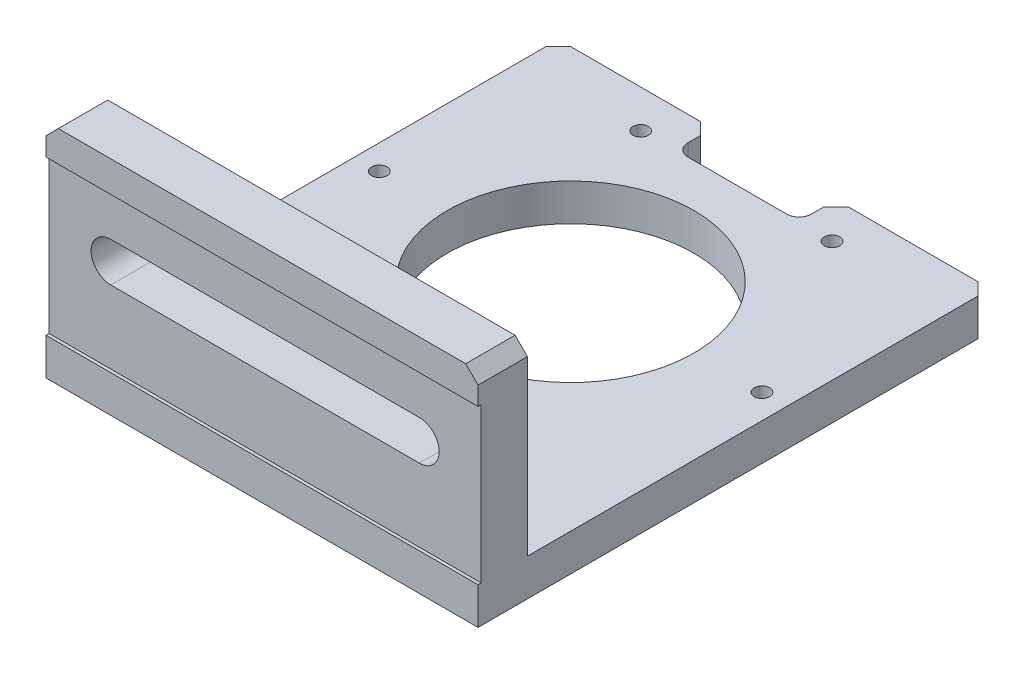
SolidWorks part; units mm, degrees
ref_plane "Front Plane" through (0, 0, 0) normal (0, 0, 1) x (1, 0, 0)
ref_plane "Top Plane" through (0, 0, 0) normal (0, 1, 0) x (1, 0, 0)
ref_plane "Right Plane" through (0, 0, 0) normal (1, 0, 0) x (0, 0, -1)
sketch "Sketch1" plane through (0, 0, 0) normal (0, 1, 0) x (1, 0, 0)
  line L1 (-35, -41.5) -> (35, -41.5)
  line L2 (-35, -41.5) -> (-35, 41.5)
  line L3 (-35, 41.5) -> (35, 41.5)
  line L4 (35, -41.5) -> (35, 41.5)
  line L5 (-35, -41.5) -> (35, 41.5) construction
  line L6 (-35, 41.5) -> (35, -41.5) construction
  point P0 (0, 0)
  dimension "D1" = 70
  dimension "D2" = 83
extrude "Boss-Extrude1" add sketch "Sketch1" along normal blind 6
sketch "Sketch2" plane through (0, 6, 0) normal (0, 1, 0) x (1, 0, 0)
  line L0 (35, -41.5) -> (35, 41.5) construction
  line L1 (-35, -41.5) -> (35, -41.5)
  line L2 (-35, -41.5) -> (-35, -33.5)
  line L3 (-35, -33.5) -> (35, -33.5)
  line L4 (35, -41.5) -> (35, -33.5)
  dimension "D1" = 8
extrude "Boss-Extrude2" add sketch "Sketch2" along normal blind 30
sketch "Sketch3" plane through (0, 0, 0) normal (0, -1, 0) x (1, 0, 0)
  line L0 (-35, 41.5) -> (35, 41.5) construction
  line L1 (-35, -41.5) -> (-35, 41.5) construction
  circle A0 centre (0, -8.5) radius 20
  dimension "D1" = 50
  dimension "D3" = 40
  dimension "D2" = 35
extrude "Cut-Extrude1" cut sketch "Sketch3" against normal blind 20
sketch "Sketch4" plane through (0, 6, 0) normal (0, 1, 0) x (1, 0, 0)
  line L0 (35, 41.5) -> (-35, 41.5) construction
  line L1 (-10, 47.5192) -> (10, 47.5192)
  line L2 (-10, 47.5192) -> (-10, 35.5)
  line L3 (-10, 35.5) -> (10, 35.5)
  line L4 (10, 47.5192) -> (10, 35.5)
  line L5 (-35, 41.5) -> (-35, -33.5) construction
  line L6 (35, -33.5) -> (35, 41.5) construction
  dimension "D1" = 6
  dimension "D2" = 25
  dimension "D3" = 25
extrude "Cut-Extrude2" cut sketch "Sketch4" against normal blind 20
sketch "Sketch5" plane through (0, 6, 0) normal (0, 1, 0) x (1, 0, 0)
  circle A0 centre (0, 8.5) radius 31 construction
  circle A1 centre (31, 8.5) radius 1.25
  circle A2 centre (15.5, -18.3468) radius 1.25
  circle A3 centre (-15.5, -18.3468) radius 1.25
  circle A4 centre (-31, 8.5) radius 1.25
  circle A5 centre (-15.5, 35.3468) radius 1.25
  circle A6 centre (15.5, 35.3468) radius 1.25
  point P18 (0, 8.5)
  dimension "D1" = 62
  dimension "D2" = 2.5
  dimension "D3" = 6
extrude "Cut-Extrude3" cut sketch "Sketch5" against normal blind 20
sketch "Sketch6" plane through (0, 0, 33.5) normal (0, 0, -1) x (-1, 0, 0)
  line L0 (25, 21) -> (-25, 21) construction
  line L1 (25, 17.8) -> (-25, 17.8)
  line L2 (25, 24.2) -> (-25, 24.2)
  line L3 (-35, 36) -> (-35, 6) construction
  line L4 (-35, 6) -> (35, 6) construction
  arc A0 (25, 17.8) -> (25, 24.2) centre (25, 21) ccw
  arc A1 (-25, 24.2) -> (-25, 17.8) centre (-25, 21) ccw
  point P2 (0, 21)
  dimension "D1" = 3.2
  dimension "D2" = 35
  dimension "D3" = 50
  dimension "D4" = 15
extrude "Cut-Extrude4" cut sketch "Sketch6" against normal blind 20
sketch "Sketch7" plane through (-35, 0, 0) normal (-1, 0, 0) x (0, 0, 1)
  line L0 (41.5, 36) -> (41.5, 0) construction
  line L1 (41.5, 6) -> (41, 6)
  line L2 (41.5, 6) -> (41.5, 31)
  line L3 (41.5, 31) -> (41, 31)
  line L4 (41, 6) -> (41, 31)
  line L5 (33.5, 36) -> (41.5, 36) construction
  dimension "D1" = 25
  dimension "D2" = 0.5
  dimension "D3" = 5
extrude "Cut-Extrude5" cut sketch "Sketch7" against normal blind 90
fillet "Fillet1" radius 2 2 edges at (-10, 3, -35.5) (10, 3, -35.5)
chamfer "Chamfer1" distance 2 angle 45 6 edges at (-35, 36, 37.5) (35, 36, 37.5) (35, 3, -41.5) (-35, 3, -41.5) (10, 3, -41.5) (-10, 3, -41.5)
